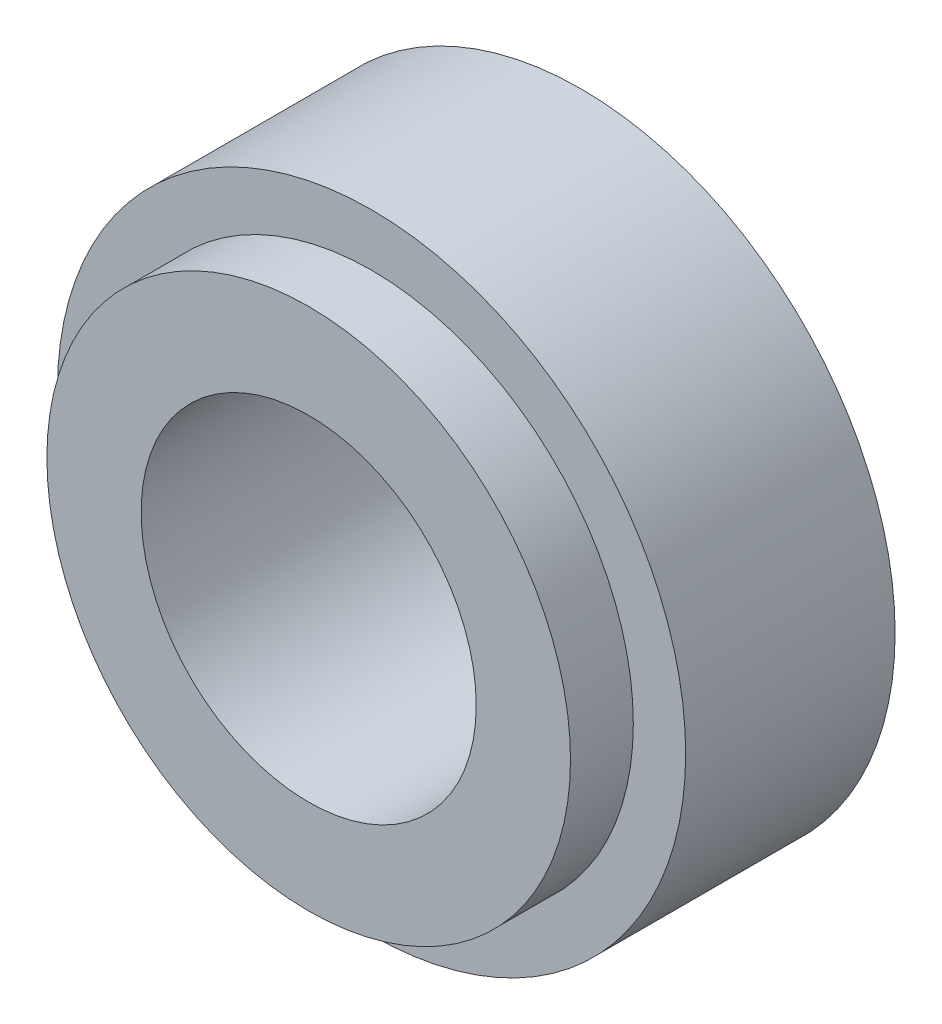
SolidWorks part; units mm, degrees
ref_plane "Front Plane" through (0, 0, 0) normal (0, 0, 1) x (1, 0, 0)
ref_plane "Top Plane" through (0, 0, 0) normal (0, 1, 0) x (1, 0, 0)
ref_plane "Right Plane" through (0, 0, 0) normal (1, 0, 0) x (0, 0, -1)
sketch "Sketch1" plane through (0, 0, 0) normal (0, 0, 1) x (1, 0, 0)
  circle A0 centre (0, 0) radius 15
  dimension "D1" = 30
extrude "Boss-Extrude1" add sketch "Sketch1" along normal blind 10
sketch "Sketch2" plane through (0, 0, 10) normal (0, 0, 1) x (1, 0, 0)
  circle A0 centre (0, 0) radius 12.5
  dimension "D1" = 25
extrude "Boss-Extrude2" add sketch "Sketch2" along normal blind 3
sketch "Sketch3" plane through (0, 0, 13) normal (0, 0, 1) x (1, 0, 0)
  circle A0 centre (0, 0) radius 8
  dimension "D1" = 16
extrude "Cut-Extrude1" cut sketch "Sketch3" against normal through all
